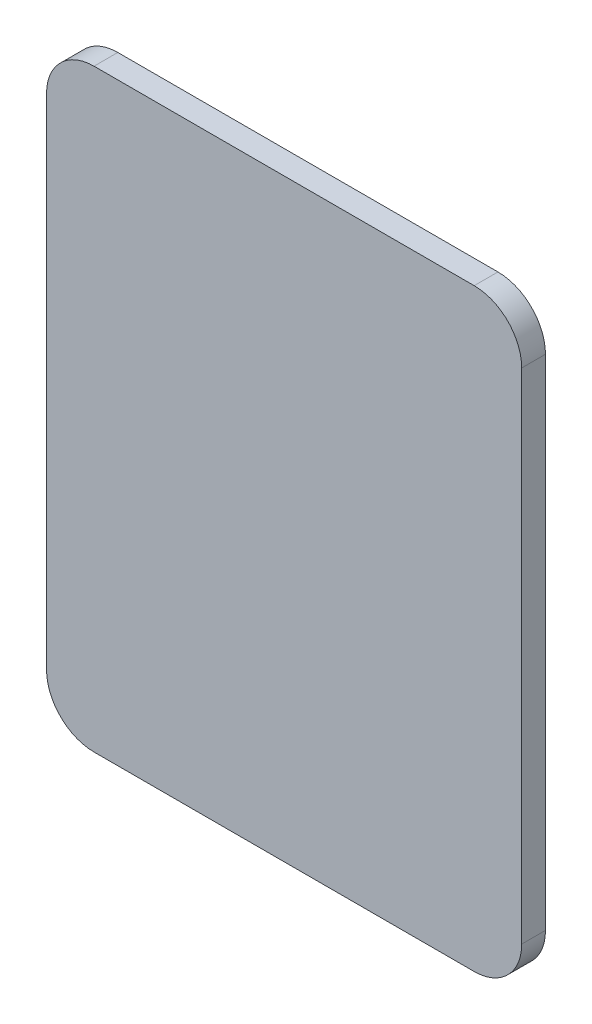
from build123d import *

# Parameters (mm, degrees)
SKETCH_1_W                   = 200
SKETCH_1_H                   = 250
EXTRUDE_1_DEPTH              = 10
FILLET_1_R                   = 20
HOLE_WIZARD_M8_2_D           = 6.8
HOLE_WIZARD_M8_2_DEPTH       = 2.957073895
HOLE_WIZARD_M8_2_CSINK_D     = 8.05
HOLE_WIZARD_M8_2_CSINK_ANGLE = 90
HOLE_WIZARD_M8_2_TIP         = 2.042926105
HOLE_WIZARD_M6_1_D           = 5
HOLE_WIZARD_M6_1_DEPTH       = 6.497848452
HOLE_WIZARD_M6_1_CSINK_D     = 6.05
HOLE_WIZARD_M6_1_CSINK_ANGLE = 90
HOLE_WIZARD_M6_1_TIP         = 1.502151548


with BuildPart() as part:
    # 草图1 → 凸台-拉伸1 (new body)
    with BuildSketch(Plane.XY):
        Rectangle(SKETCH_1_W, SKETCH_1_H)
    extrude(amount=EXTRUDE_1_DEPTH)

    # 圆角1
    fillet_1_edges = [part.edges().sort_by_distance(p)[0] for p in [
        (-100, 125, 5),
        (100, 125, 5),
        (100, -125, 5),
        (-100, -125, 5),
    ]]
    fillet(fillet_1_edges, radius=FILLET_1_R)

    # M8 螺纹孔2
    with Locations(Plane(origin=(0, 0, 0), x_dir=(-1, 0, 0), z_dir=(0, 0, -1))):
        with Locations((25, -100), (25, -65), (-25, -65), (-25, -100), (25, 100), (25, 65), (-25, 65), (-25, 100)):
            CounterSinkHole(HOLE_WIZARD_M8_2_D / 2, HOLE_WIZARD_M8_2_CSINK_D / 2, depth=HOLE_WIZARD_M8_2_DEPTH, counter_sink_angle=HOLE_WIZARD_M8_2_CSINK_ANGLE)
            with Locations((0, 0, -(HOLE_WIZARD_M8_2_DEPTH + HOLE_WIZARD_M8_2_TIP / 2))):  # 118° drill point
                Cone(0, HOLE_WIZARD_M8_2_D / 2, HOLE_WIZARD_M8_2_TIP, mode=Mode.SUBTRACT)

    # M6 螺纹孔1
    with Locations(Plane(origin=(0, 0, 0), x_dir=(-1, 0, 0), z_dir=(0, 0, -1))):
        with Locations((70, 20), (30, 20), (70, -20), (30, -20), (-30, 20), (-30, -20), (-70, 20), (-70, -20)):
            CounterSinkHole(HOLE_WIZARD_M6_1_D / 2, HOLE_WIZARD_M6_1_CSINK_D / 2, depth=HOLE_WIZARD_M6_1_DEPTH, counter_sink_angle=HOLE_WIZARD_M6_1_CSINK_ANGLE)
            with Locations((0, 0, -(HOLE_WIZARD_M6_1_DEPTH + HOLE_WIZARD_M6_1_TIP / 2))):  # 118° drill point
                Cone(0, HOLE_WIZARD_M6_1_D / 2, HOLE_WIZARD_M6_1_TIP, mode=Mode.SUBTRACT)


solid = part.part
